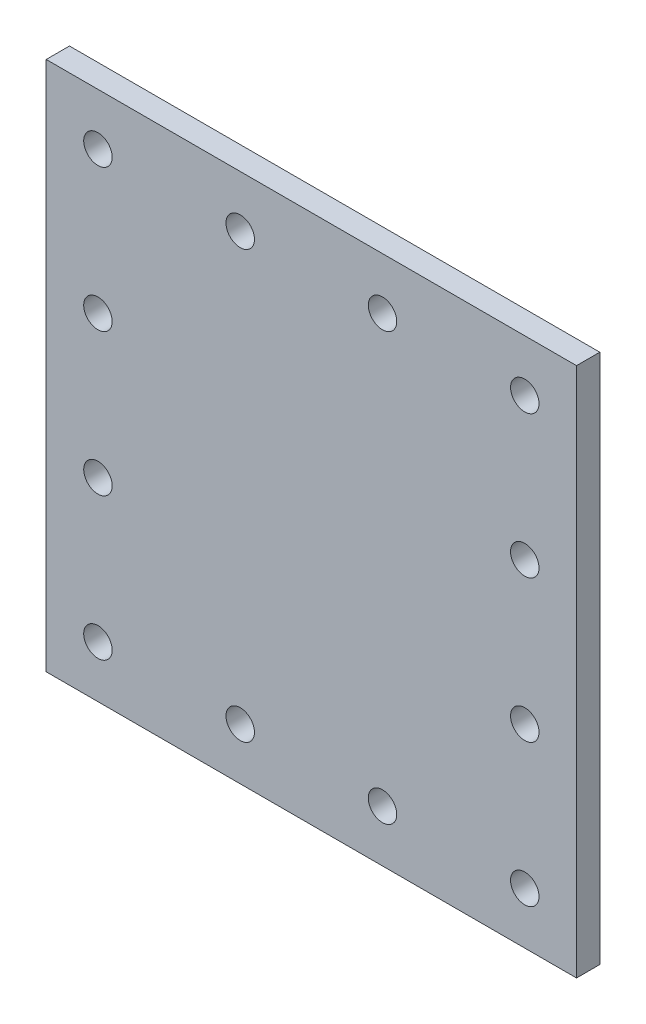
from build123d import *

# Parameters (mm, degrees)
SKETCH1_W           = 410
SKETCH1_H           = 410
BOSS_EXTRUDE1_DEPTH = 18
SKETCH2_R           = 11
CUT_EXTRUDE1_DEPTH  = 18


with BuildPart() as part:
    # Sketch1 → Boss-Extrude1 (new body)
    with BuildSketch(Plane.XY):
        Rectangle(SKETCH1_W, SKETCH1_H)
    extrude(amount=BOSS_EXTRUDE1_DEPTH)

    # Sketch2 → Cut-Extrude1 (cut)
    with BuildSketch(Plane.XY.offset(18)):
        with Locations((-165, 165)):
            Circle(SKETCH2_R)
        with Locations((165, 165)):
            Circle(SKETCH2_R)
        with Locations((165, -165)):
            Circle(SKETCH2_R)
        with Locations((-165, -165)):
            Circle(SKETCH2_R)
        with Locations((-165, 55)):
            Circle(SKETCH2_R)
        with Locations((-165, -55)):
            Circle(SKETCH2_R)
        with Locations((-55, 165)):
            Circle(SKETCH2_R)
        with Locations((55, 165)):
            Circle(SKETCH2_R)
        with Locations((165, 55)):
            Circle(SKETCH2_R)
        with Locations((165, -55)):
            Circle(SKETCH2_R)
        with Locations((-55, -165)):
            Circle(SKETCH2_R)
        with Locations((55, -165)):
            Circle(SKETCH2_R)
    extrude(amount=-CUT_EXTRUDE1_DEPTH, mode=Mode.SUBTRACT)


solid = part.part
